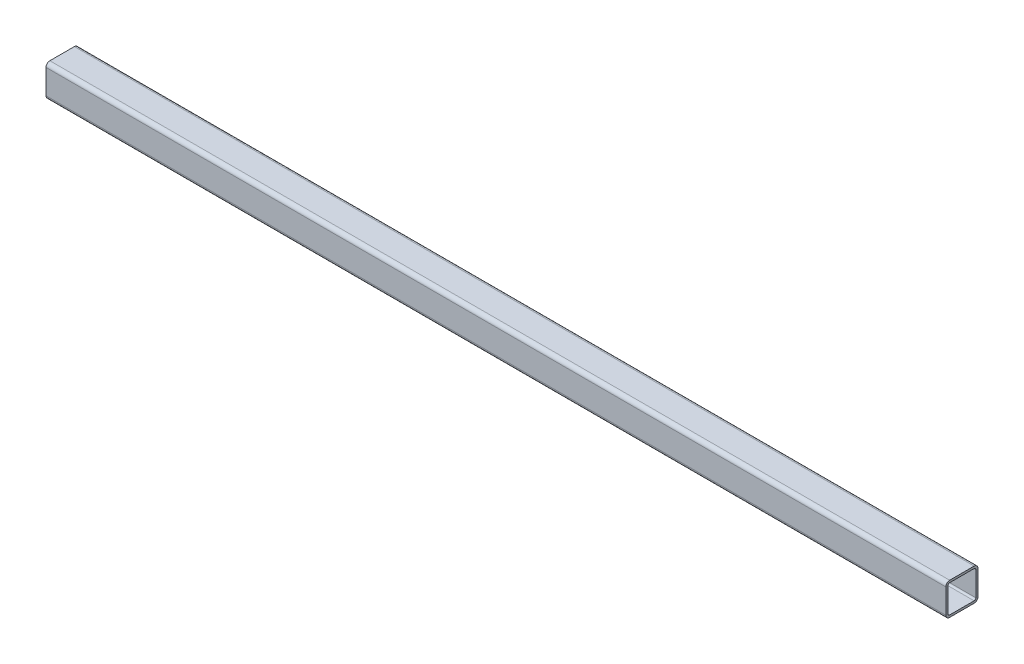
from build123d import *

# Parameters (mm, degrees)
MEMBER_30_2_1_DEPTH = 838


with BuildPart() as part:
    # Sketch1 → Member 30_2_1 (new body)
    with BuildSketch(Plane(origin=(-419, 0, 0), x_dir=(0, 0, -1), z_dir=(1, 0, 0))):
        with BuildLine():
            Line((-11.4, -15), (11.4, -15))
            ThreePointArc((11.4, -15), (13.945584412, -13.945584412), (15, -11.4))
            Line((15, -11.4), (15, 11.4))
            ThreePointArc((15, 11.4), (13.945584412, 13.945584412), (11.4, 15))
            Line((11.4, 15), (-11.4, 15))
            ThreePointArc((-11.4, 15), (-13.945584412, 13.945584412), (-15, 11.4))
            Line((-15, 11.4), (-15, -11.4))
            ThreePointArc((-15, -11.4), (-13.945584412, -13.945584412), (-11.4, -15))
        make_face()
        with BuildLine():
            Line((-11.4, -13), (11.4, -13))
            ThreePointArc((11.4, -13), (12.53137085, -12.53137085), (13, -11.4))
            Line((13, -11.4), (13, 11.4))
            ThreePointArc((13, 11.4), (12.53137085, 12.53137085), (11.4, 13))
            Line((11.4, 13), (-11.4, 13))
            ThreePointArc((-11.4, 13), (-12.53137085, 12.53137085), (-13, 11.4))
            Line((-13, 11.4), (-13, -11.4))
            ThreePointArc((-13, -11.4), (-12.53137085, -12.53137085), (-11.4, -13))
        make_face(mode=Mode.SUBTRACT)
    extrude(amount=MEMBER_30_2_1_DEPTH)


solid = part.part
